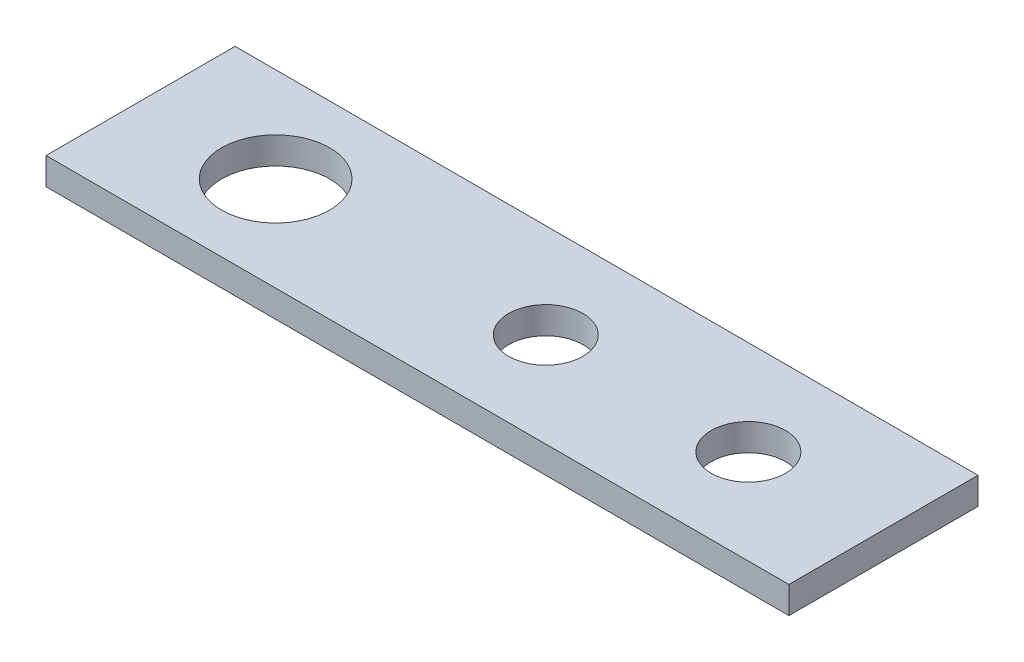
from build123d import *

# Parameters (mm, degrees)
EXTRUDE_1_DEPTH      = 1
EXTRUDE_1_DEPTH_BACK = 1
SKETCH_1_W           = 55
SKETCH_1_H           = 14
SKETCH_1_R           = 2.75
SKETCH_1_R_2         = 4


with BuildPart() as part:
    # 草图1 → 凸台-拉伸1 (new, two sides: drawn at the far end of the back side and taken through both)
    with BuildSketch(Plane(origin=(0, 0, 0), x_dir=(1, 0, 0), z_dir=(0, 1, 0)).offset(-EXTRUDE_1_DEPTH_BACK)):
        with Locations((17.5, 0)):
            Rectangle(SKETCH_1_W, SKETCH_1_H)
        with Locations(Location((35, 0, 0), (0, 0, 270))):
            Circle(SKETCH_1_R, mode=Mode.SUBTRACT)
        with Locations(Location((20, 0, 0), (0, 0, 270))):
            Circle(SKETCH_1_R, mode=Mode.SUBTRACT)
        with Locations(Location((0, 0, 0), (0, 0, 270))):
            Circle(SKETCH_1_R_2, mode=Mode.SUBTRACT)
    extrude(amount=EXTRUDE_1_DEPTH + EXTRUDE_1_DEPTH_BACK)


solid = part.part
